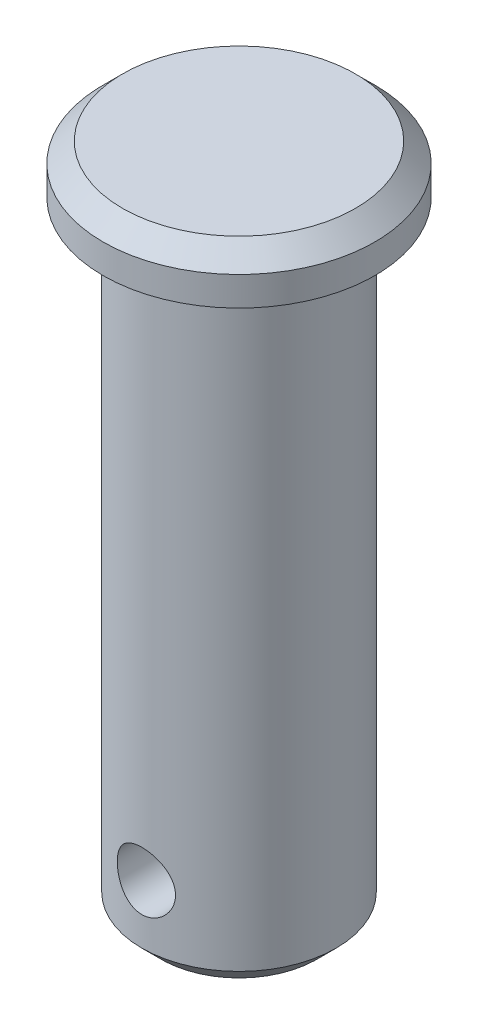
SolidWorks part; units mm, degrees
material "45"
ref_plane "前视基准面" through (0, 0, 0) normal (0, 0, 1) x (1, 0, 0)
ref_plane "上视基准面" through (0, 0, 0) normal (0, 1, 0) x (1, 0, 0)
ref_plane "右视基准面" through (0, 0, 0) normal (1, 0, 0) x (0, 0, -1)
sketch "草图1" plane through (0, 0, 0) normal (0, 1, 0) x (1, 0, 0)
  circle A0 centre (0, 0) radius 7
  dimension "D1" = 14
extrude "凸台-拉伸1" add sketch "草图1" along normal blind 2.5
sketch "草图2" plane through (0, 0, 0) normal (0, -1, 0) x (1, 0, 0)
  circle A0 centre (0, 0) radius 5
  dimension "D1" = 10
extrude "凸台-拉伸2" add sketch "草图2" along normal blind 32
ref_plane "基准面1" through (-5, 0, 0) normal (-1, 0, 0) x (0, 0, 1)
chamfer "倒角1" distance 1 angle 45 2 edges at (0, -32, -5) (0, 2.5, 7)
sketch "草图10" plane through (0, 0, 0) normal (0, 0, 1) x (1, 0, 0)
  line L0 (-4, -32) -> (4, -32) construction
  circle A0 centre (0, -28) radius 1.5
  dimension "D1" = 3
  dimension "D2" = 4
extrude "切除-拉伸2" cut sketch "草图10" against normal through all both and the other way through all
fillet "圆角1" radius 0.5 1 edges at (0, 0, -5)
